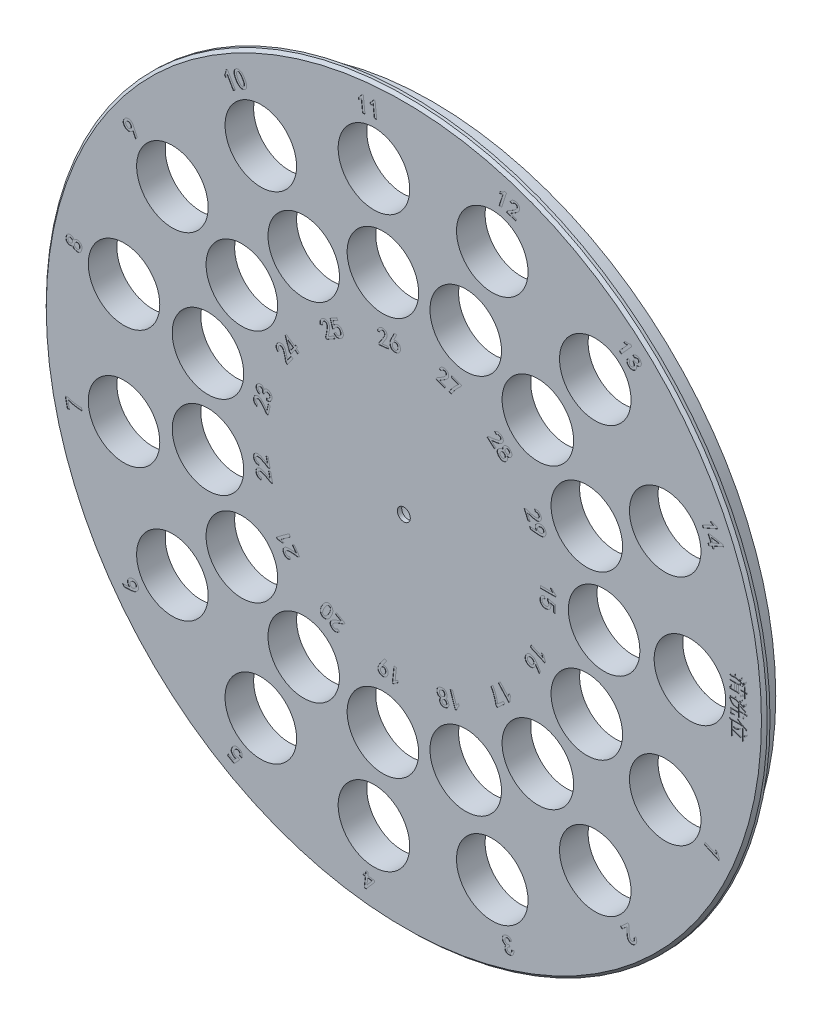
SolidWorks part; units mm, degrees
material "ABS"
ref_plane "Front Plane" through (0, 0, 0) normal (0, 0, 1) x (1, 0, 0)
ref_plane "Top Plane" through (0, 0, 0) normal (0, 1, 0) x (1, 0, 0)
ref_plane "Right Plane" through (0, 0, 0) normal (1, 0, 0) x (0, 0, -1)
sketch "Sketch1" plane through (0, 0, 0) normal (0, 0, 1) x (1, 0, 0)
  circle A0 centre (0, 0) radius 126
  dimension "D1" = 252
extrude "Boss-Extrude1" add sketch "Sketch1" along normal blind 2
sketch "Sketch3" plane through (0, 0, 0) normal (0, 0, -1) x (-1, 0, 0)
  circle A1 centre (0, 0) radius 120
  dimension "D2" = 240
extrude "Boss-Extrude3" add sketch "Sketch3" along normal blind 8
sketch "Sketch8" plane through (0, 0, 0) normal (0, 0, -1) x (-1, 0, 0)
  circle A0 centre (0, 0) radius 2.25
  dimension "D1" = 4.5
extrude "Cut-Extrude3" cut sketch "Sketch8" against normal blind 8.5
sketch "Sketch2" plane through (0, 0, 2) normal (0, 0, 1) x (1, 0, 0)
  line L0 (-126, 0) -> (126, 0) construction
  line L1 (0, 126) -> (0, -126) construction
  line L2 (0, 0) -> (115.1067, -51.2488) construction
  line L3 (0, 0) -> (84.3105, -93.6362) construction
  line L4 (0, 0) -> (38.9361, -119.8331) construction
  line L5 (0, 0) -> (-13.1706, -125.3098) construction
  line L6 (0, 0) -> (-63, -109.1192) construction
  line L7 (0, 0) -> (-101.9361, -74.0609) construction
  line L8 (0, 0) -> (-123.2466, -26.1969) construction
  line L9 (0, 0) -> (-123.2466, 26.1969) construction
  line L10 (0, 0) -> (-101.9361, 74.0609) construction
  line L11 (0, 0) -> (-63, 109.1192) construction
  line L12 (0, 0) -> (-13.1706, 125.3098) construction
  line L13 (0, 0) -> (38.9361, 119.8331) construction
  line L14 (0, 0) -> (84.3105, 93.6362) construction
  line L15 (0, 0) -> (115.1067, 51.2488) construction
  line L16 (0, 0) -> (126, 0) construction
  circle A0 centre (0, 0) radius 126 construction
  circle A1 centre (0, 0) radius 100 construction
  circle A2 centre (100, 0) radius 12.5
  circle A3 centre (0, 0) radius 70 construction
  circle A4 centre (91.3545, -40.6737) radius 12.5
  circle A6 centre (66.9131, -74.3145) radius 12.5
  circle A8 centre (30.9017, -95.1057) radius 12.5
  circle A10 centre (-10.4528, -99.4522) radius 12.5
  circle A11 centre (70, 0) radius 12.5
  circle A12 centre (-50, -86.6025) radius 12.5
  circle A13 centre (63.9482, -28.4716) radius 12.5
  circle A14 centre (-80.9017, -58.7785) radius 12.5
  circle A15 centre (46.8391, -52.0201) radius 12.5
  circle A16 centre (-97.8148, -20.7912) radius 12.5
  circle A17 centre (21.6312, -66.574) radius 12.5
  circle A18 centre (-97.8148, 20.7912) radius 12.5
  circle A19 centre (-7.317, -69.6165) radius 12.5
  circle A20 centre (-80.9017, 58.7785) radius 12.5
  circle A21 centre (-35, -60.6218) radius 12.5
  circle A22 centre (-50, 86.6025) radius 12.5
  circle A23 centre (-56.6312, -41.145) radius 12.5
  circle A24 centre (-10.4528, 99.4522) radius 12.5
  circle A25 centre (-68.4703, -14.5538) radius 12.5
  circle A26 centre (30.9017, 95.1057) radius 12.5
  circle A27 centre (-68.4703, 14.5538) radius 12.5
  circle A28 centre (66.9131, 74.3145) radius 12.5
  circle A29 centre (-56.6312, 41.145) radius 12.5
  circle A30 centre (91.3545, 40.6737) radius 12.5
  circle A31 centre (-35, 60.6218) radius 12.5
  circle A32 centre (-7.317, 69.6165) radius 12.5
  circle A33 centre (21.6312, 66.574) radius 12.5
  circle A34 centre (46.8391, 52.0201) radius 12.5
  circle A35 centre (63.9482, 28.4716) radius 12.5
  point P81 (0, 0)
  point P88 (0, 0)
  point P131 (0, 0)
  dimension "D1" = 30
  dimension "D2" = 25
  dimension "D3" = 15
  dimension "D4" = 100
  dimension "D6" = 24
  dimension "D5" = 15
  dimension "D7" = 15
extrude "Cut-Extrude1" cut sketch "Sketch2" against normal through all
hole_wizard "M4 Tapped Hole1" positions "Sketch19" profile "Sketch20" tap size "M4" standard "GB"
sketch "Sketch19" plane through (0, 0, -8) normal (0, 0, -1) x (-1, 0, 0)
  line L3 (10.4528, 99.4522) -> (50, 86.6025) construction
  line L5 (30.2264, 93.0274) -> (32.1378, 98.9099) construction
  circle A0 centre (0, 0) radius 104 construction
  point P0 (32.1378, 98.9099)
  point P39 (104, 0)
  point P40 (32.1378, -98.9099)
  point P41 (-84.1378, -61.1297)
  point P42 (-84.1378, 61.1297)
  point P43 (0, 0)
  dimension "D1" = 208
  dimension "D2" = 5
cosmetic thread "Cosmetic Thread5" parameters "D1"=5, "D2"=4
sketch "Sketch20" plane through (-32.1378, 98.9099, -8) normal (1, 0, 0) x (0, 1, 0)
  line L0 (0, 0) -> (0, 8.9914)
  line L1 (0, 8.9914) -> (1.65, 8)
  line L2 (1.65, 8) -> (1.65, 0)
  line L5 (1.65, 0) -> (0, 0)
  line L10 (0, 8.9914) -> (-1.65, 8) construction
  line L11 (0, -6.35) -> (0, 107.95) construction
  dimension "螺纹孔钻头直径" = 3.3
  dimension "螺纹孔钻头深度" = 8
  dimension "导头角度" = 118
cosmetic thread "Cosmetic Thread6" parameters "D1"=5, "D2"=4
cosmetic thread "Cosmetic Thread7" parameters "D1"=5, "D2"=4
cosmetic thread "Cosmetic Thread8" parameters "D1"=5, "D2"=4
cosmetic thread "Cosmetic Thread9" parameters "D1"=5, "D2"=4
cosmetic thread "Cosmetic Thread10" parameters "D1"=5, "D2"=4
chamfer "Chamfer1" distance 1 angle 45 1 edges at (126, 0, 2)
sketch "Sketch26" plane through (0, 0, -8) normal (0, 0, -1) x (-1, 0, 0)
  line L0 (0, 0) -> (-100, 0) construction
  line L1 (0, 0) -> (-50, 0) construction
  line L2 (-10.6213, -4.5) -> (-50, -4.5)
  line L3 (-10.6213, 4.5) -> (-50, 4.5)
  arc A0 (-10.6213, 4.5) -> (-6.8945, 6.1667) centre (-10.6213, 9.5) ccw
  arc A1 (-6.8945, -6.1667) -> (-6.8945, 6.1667) centre (0, 0) ccw
  arc A4 (-50, 4.5) -> (-50, -4.5) centre (-50, 0) ccw
  arc A5 (-10.6213, -4.5) -> (-6.8945, -6.1667) centre (-10.6213, -9.5) cw
  point P4 (-25, 0)
  point P6 (0, 0)
  dimension "D1" = 18.5
  dimension "D6" = 5
  dimension "D2" = 9
  dimension "D3" = 50
  dimension "D4" = 25
extrude "Cut-Extrude4" cut sketch "Sketch26" against normal offset from surface (8.5 mm away) 1.5 up to face at (125, 0, 2)
sketch "Sketch27" plane through (0, 0, 2) normal (0, 0, 1) x (1, 0, 0)
  line L0 (0, 0) -> (47.5, 10.0964) construction
  line L1 (115, -24.444) -> (115, 24.444) construction
  line L2 (115, 24.444) -> (95.1155, 69.1054) construction
  line L3 (95.1155, 69.1054) -> (58.7846, 101.8179) construction
  line L4 (58.7846, 101.8179) -> (12.2893, 116.9251) construction
  line L5 (12.2893, 116.9251) -> (-36.3309, 111.8149) construction
  line L6 (-36.3309, 111.8149) -> (-78.6691, 87.3709) construction
  line L7 (-78.6691, 87.3709) -> (-107.4048, 47.8197) construction
  line L8 (-107.4048, 47.8197) -> (-117.5692, 0) construction
  line L9 (-117.5692, 0) -> (-107.4048, -47.8197) construction
  line L10 (-107.4048, -47.8197) -> (-78.6691, -87.3709) construction
  line L11 (-78.6691, -87.3709) -> (-36.3309, -111.8149) construction
  line L12 (-36.3309, -111.8149) -> (12.2893, -116.9251) construction
  line L13 (12.2893, -116.9251) -> (58.7846, -101.8179) construction
  line L14 (58.7846, -101.8179) -> (95.1155, -69.1054) construction
  line L15 (95.1155, -69.1054) -> (115, -24.444) construction
  line L16 (0, 0) -> (115, 0) construction
  line L17 (47.5, 10.0964) -> (39.2868, 28.5435) construction
  line L18 (39.2868, 28.5435) -> (24.2806, 42.0552) construction
  line L19 (24.2806, 42.0552) -> (5.076, 48.2952) construction
  line L20 (5.076, 48.2952) -> (-15.0062, 46.1844) construction
  line L21 (-15.0062, 46.1844) -> (-32.4938, 36.088) construction
  line L22 (-32.4938, 36.088) -> (-44.3628, 19.7516) construction
  line L23 (-44.3628, 19.7516) -> (-48.5612, 0) construction
  line L24 (-48.5612, 0) -> (-44.3628, -19.7516) construction
  line L25 (-44.3628, -19.7516) -> (-32.4938, -36.088) construction
  line L26 (-32.4938, -36.088) -> (-15.0062, -46.1844) construction
  line L27 (-15.0062, -46.1844) -> (5.076, -48.2952) construction
  line L28 (5.076, -48.2952) -> (24.2806, -42.0552) construction
  line L29 (24.2806, -42.0552) -> (39.2868, -28.5435) construction
  line L30 (39.2868, -28.5435) -> (47.5, -10.0964) construction
  line L31 (47.5, -10.0964) -> (47.5, 10.0964) construction
  circle A0 centre (0, 0) radius 115 construction
  circle A2 centre (0, 0) radius 47.5 construction
  text T0 "清洗位" font "华文宋体" height in points 15
  text T1 "1" font "黑体" height in points 18
  text T2 "2" font "黑体" height in points 18
  text T3 "3" font "黑体" height in points 18
  text T4 "4" font "黑体" height in points 18
  text T5 "5" font "黑体" height in points 18
  text T6 "6" font "黑体" height in points 18
  text T7 "7" font "黑体" height in points 18
  text T8 "8" font "黑体" height in points 18
  text T9 "9" font "黑体" height in points 18
  text T10 "10" font "黑体" height in points 18
  text T11 "11" font "黑体" height in points 18
  text T12 "12" font "黑体" height in points 18
  text T13 "13" font "黑体" height in points 18
  text T14 "14" font "黑体" height in points 18
  text T15 "29" font "@黑体" height in points 18
  text T16 "15" font "黑体" height in points 18
  text T17 "16" font "黑体" height in points 18
  text T18 "17" font "黑体" height in points 18
  text T19 "18" font "黑体" height in points 18
  text T20 "19" font "黑体" height in points 18
  text T21 "20" font "黑体" height in points 18
  text T22 "21" font "黑体" height in points 18
  text T23 "22" font "黑体" height in points 18
  text T24 "23" font "黑体" height in points 18
  text T25 "24" font "黑体" height in points 18
  text T26 "25" font "黑体" height in points 18
  text T27 "26" font "黑体" height in points 18
  text T28 "27" font "黑体" height in points 18
  text T29 "28" font "黑体" height in points 18
  dimension "D1" = 95
  dimension "D2" = 230
  dimension "D3" = 12
extrude "Cut-Extrude5" cut sketch "Sketch27" against normal blind 0.1
